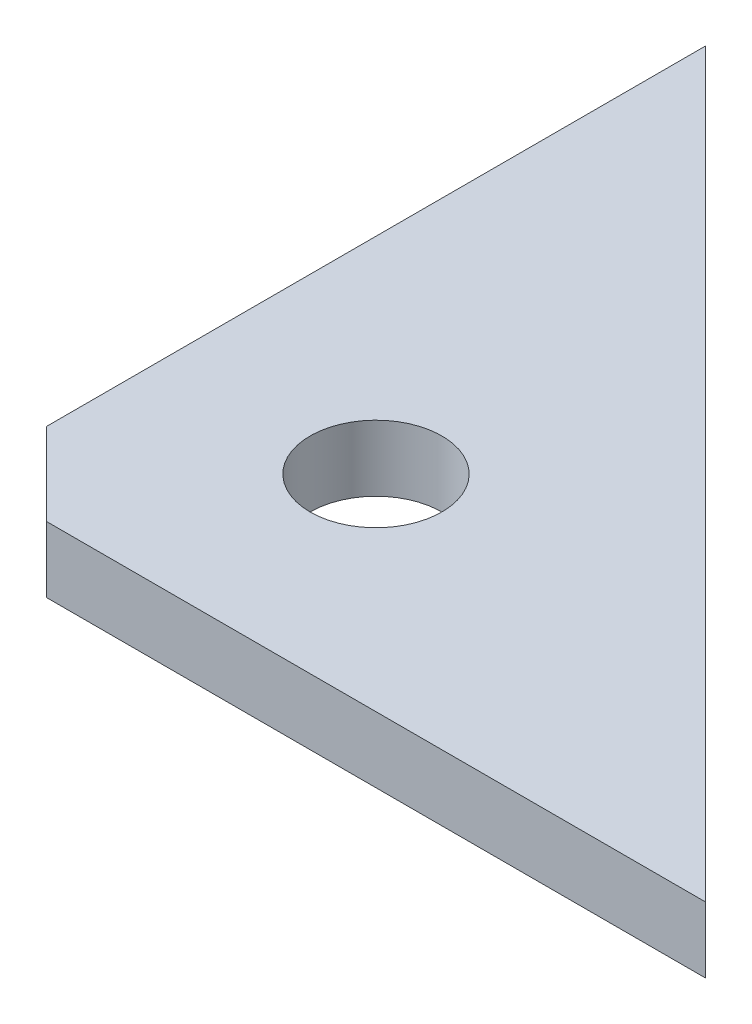
from build123d import *

# Parameters (mm, degrees)
EXTRUDE_1_DEPTH         = 8
CHAMFER_1_SIZE          = 10
HOLE_WIZARD_16_0_16_1_D = 16


with BuildPart() as part:
    # 草图1 → 凸台-拉伸1 (new body)
    with BuildSketch(Plane(origin=(0, 0, 0), x_dir=(1, 0, 0), z_dir=(0, 1, 0))):
        Polygon((0, 0), (0, 90), (90, 0), align=None)
    extrude(amount=EXTRUDE_1_DEPTH)

    # 倒角1
    chamfer_1_edges = [part.edges().sort_by_distance(p)[0] for p in [
        (0, 4, 0),
    ]]
    chamfer(chamfer_1_edges, length=CHAMFER_1_SIZE)

    # Ø16.0 (16) 直径孔1 (through all)
    with Locations(Plane(origin=(0, 8, 0), x_dir=(1, 0, 0), z_dir=(0, 1, 0))):
        with Locations((25, 25)):
            Hole(HOLE_WIZARD_16_0_16_1_D / 2)


solid = part.part
